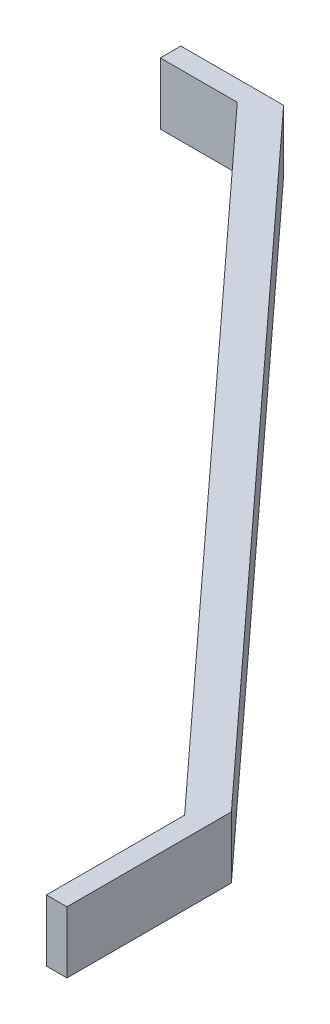
SolidWorks part; units mm, degrees
material "AISI 304"
ref_plane "Front Plane" through (0, 0, 0) normal (0, 0, 1) x (1, 0, 0)
ref_plane "Top Plane" through (0, 0, 0) normal (0, 1, 0) x (1, 0, 0)
ref_plane "Right Plane" through (0, 0, 0) normal (1, 0, 0) x (0, 0, -1)
sketch "Sketch1" plane through (0, 500, 0) normal (0, -1, 0) x (1, 0, 0)
  line L0 (376.6665, 456.2997) -> (376.6665, 416.2997)
  line L1 (376.6665, 416.2997) -> (234.1665, 261.0997)
  line L2 (209.1665, 261.0997) -> (426.6665, 261.0997) construction
  line L3 (361.8709, 412.0141) -> (227.8966, 266.0997)
  line L5 (376.6665, 416.2997) -> (26.6665, 416.2997) construction
  line L6 (376.6665, 416.2997) -> (376.6665, 466.2997) construction
  line L7 (376.6665, 456.2997) -> (371.6665, 456.2997)
  line L8 (371.6665, 456.2997) -> (371.6665, 422.6827)
  line L9 (361.8709, 412.0141) -> (371.6665, 422.6827)
  line L10 (209.1665, 261.0997) -> (234.1665, 261.0997)
  line L11 (209.1665, 261.0997) -> (209.1665, 266.0997)
  line L12 (209.1665, 266.0997) -> (227.8966, 266.0997)
  dimension "D1" = 8
  dimension "D2" = 40
  dimension "D3" = 5
  dimension "D4" = 25
  dimension "D5" = 5
extrude "Boss-Extrude1" add sketch "Sketch1" against normal blind 15
